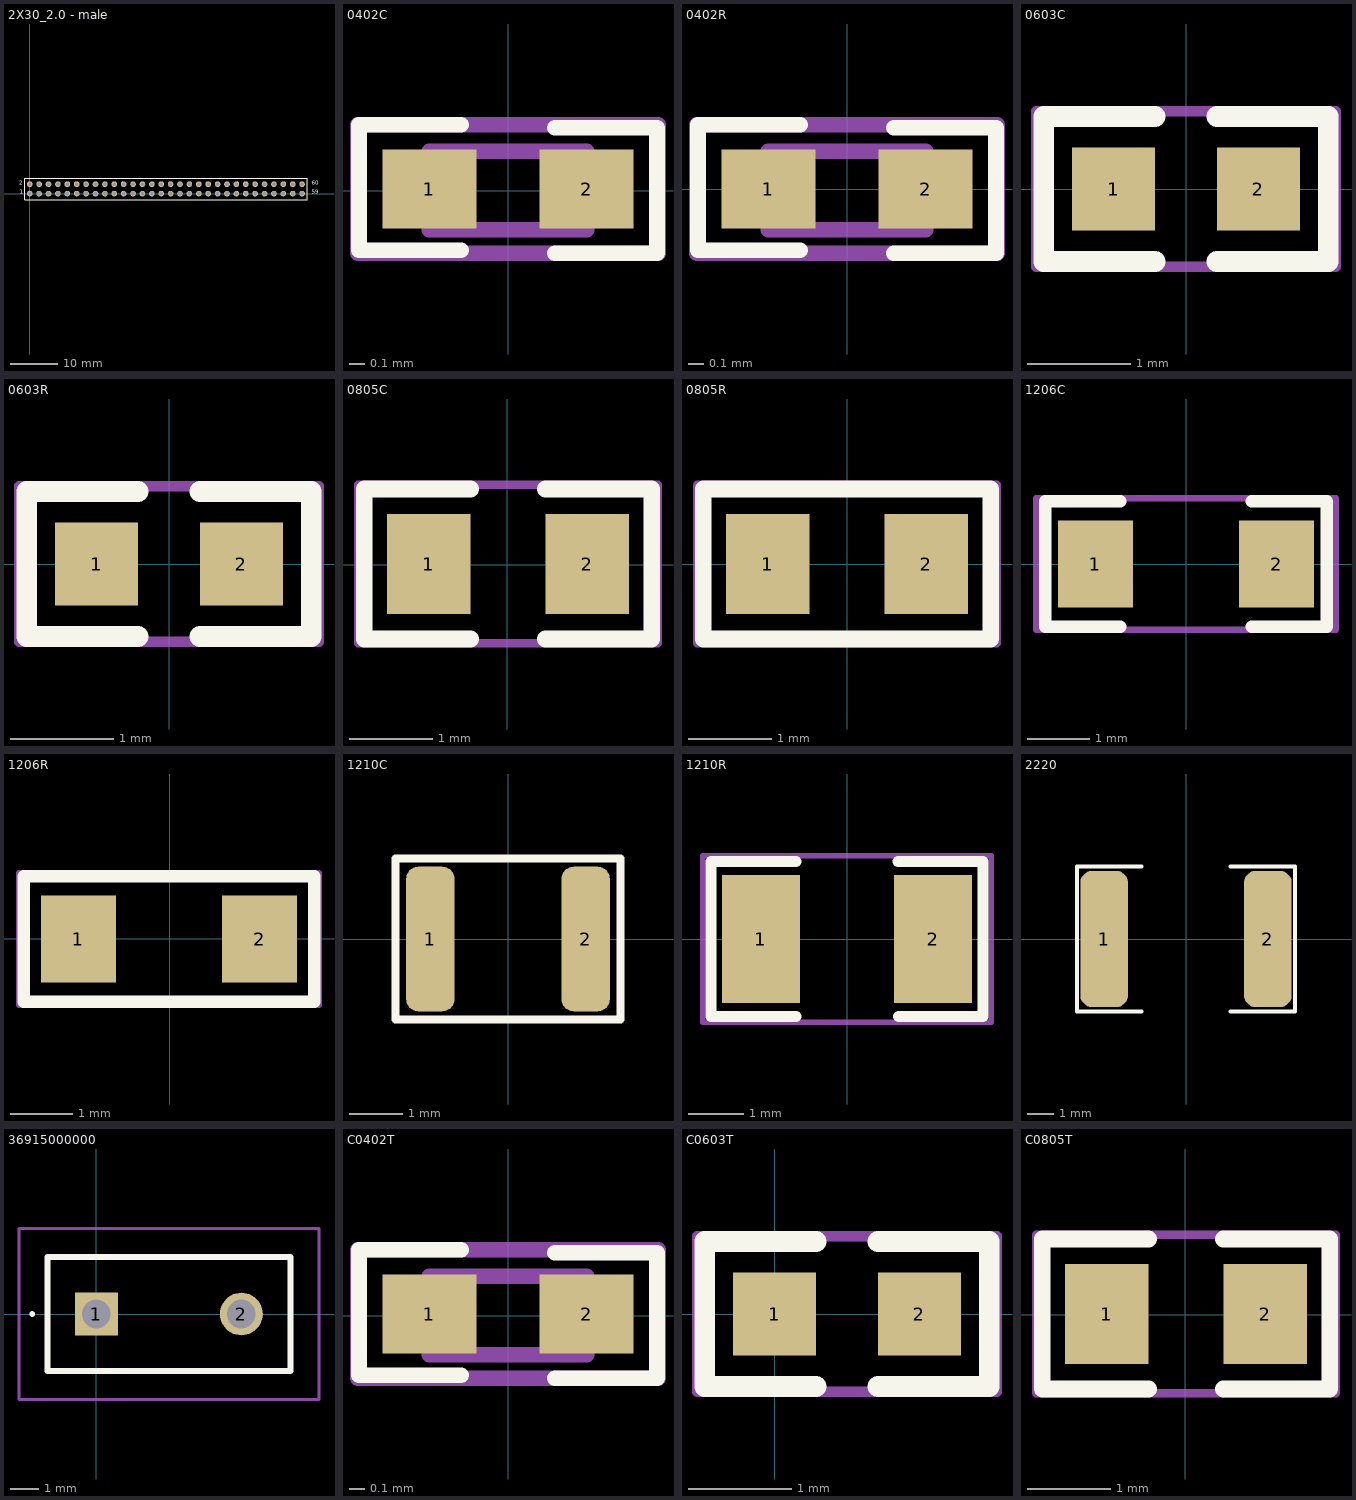
[diagram p0: the footprints below, top view; thin cyan lines are the x and y axes]
# Altium footprint library MISC82254-2.PcbLib: 93 footprints (part 1 of 6)
Each footprint in its own frame and in the unit in brackets; x right, y up, seen from the top. Pads: shape width x height; smd on the part's side, far side on the other; paste and mask are expansions set on the pad; w line width, h text height; cw(c..) or ccw(c..) is an arc to the next point about the centre after c.

## 2X30_2.0 - male [mm]
pads (60):
  round 1.2 hole 0.8: 1(0,0) 2(0,2) 3(2,0) 4(2,2) 5(4,0) 6(4,2) 7(6,0) 8(6,2) 9(8,0) 10(8,2) 11(10,0) 12(10,2) 13(12,0) 14(12,2) 15(14,0) 16(14,2) 17(16,0) 18(16,2) 19(18,0) 20(18,2) 21(20,0) 22(20,2) 23(22,0) 24(22,2) 25(24,0) 26(24,2) 27(26,0) 28(26,2) 29(28,0) 30(28,2) 31(30,0) 32(30,2) 33(32,0) 34(32,2) 35(34,0) 36(34,2) 37(36,0) 38(36,2) 39(38,0) 40(38,2) 41(40,0) 42(40,2) 43(42,0) 44(42,2) 45(44,0) 46(44,2) 47(46,0) 48(46,2) 49(48,0) 50(48,2) 51(50,0) 52(50,2) 53(52,0) 54(52,2) 55(54,0) 56(54,2) 57(56,0) 58(56,2) 59(58,0) 60(58,2)
Top Overlay:
  lines w0.254: -1.099,-1.308 -1.099,3.264 59.099,3.264 59.099,-1.308 -1.099,-1.308
  text "1" at -2.159,-0.381 h1.52
  text "2" at -2.286,1.524 h1.52
  text "60" at 60.071,1.524 h1.52
  text "59" at 60.071,-0.381 h1.52
3D body "HDR2.0-LI-2x15P.STEP": height 2.8, standoff -6.5, extent -1,-1 29,3
3D body "HDR2.0-LI-2x15P.STEP": height 2.8, standoff -6.5, extent 29,-1 59,3

## 0402C [mm]
pads (2):
  rect 0.6x0.5 smd mask+0.05: 1(-0.5,0.01) 2(0.5,0.01)
Top Overlay:
  lines w0.1: -0.298,-0.381 -0.949,-0.381 -0.949,0.419 -0.298,0.419 ; 0.298,-0.4 0.949,-0.4 0.949,0.4 0.298,0.4
Mechanical 13:
  lines w0.1: -0.5,-0.25 -0.5,0.25 0.5,0.25 0.5,-0.25 -0.5,-0.25
Mechanical 15:
  lines w0.1: -0.955,-0.4 0.955,-0.4 0.955,0.4 ; -0.955,-0.381 -0.955,0.419 0.955,0.419
3D body "GRM155R60G225ME15D.stp": height 0.55, standoff 0, extent -0.5,-0.25 0.5,0.25

## 0402R [mm]
pads (2):
  rect 0.6x0.5 smd mask+0.05: 1(-0.5,0) 2(0.5,0)
Top Overlay:
  lines w0.1: -0.298,-0.39 -0.949,-0.39 -0.949,0.41 -0.298,0.41 ; 0.298,-0.41 0.949,-0.41 0.949,0.39 0.298,0.39
Mechanical 13:
  lines w0.1: -0.5,-0.26 0.5,-0.26 0.5,0.24 -0.5,0.24 -0.5,-0.26
Mechanical 15:
  lines w0.1: -0.955,-0.41 0.955,-0.41 0.955,0.39 ; -0.955,-0.39 -0.955,0.41 0.955,0.41
3D body "CPF0402B100KE.stp": height 0.35, standoff 0, extent -0.5,-0.25 0.5,0.25

## 0603C [mm]
pads (2):
  rect 0.8x0.8 smd: 1(-0.7,0) 2(0.7,0)
Top Overlay:
  lines w0.2: -0.3,-0.7 -1.375,-0.7 -1.375,0.7 -0.3,0.7 ; 0.3,-0.7 1.375,-0.7 1.375,0.7 0.3,0.7
Mechanical 15:
  lines w0.1: -1.45,-0.75 1.45,-0.75 1.45,0.75 -1.45,0.75 -1.45,-0.75
3D body "C0603.step": height 0.8, standoff 0, extent -0.8,-0.4 0.8,0.4

## 0603R [mm]
pads (2):
  rect 0.8x0.8 smd: 1(-0.7,0) 2(0.7,0)
Top Overlay:
  lines w0.2: -0.3,-0.7 -1.375,-0.7 -1.375,0.7 -0.3,0.7 ; 0.3,-0.7 1.375,-0.7 1.375,0.7 0.3,0.7
Mechanical 15:
  lines w0.1: -1.45,-0.75 -1.45,0.75 1.45,0.75 1.45,-0.75 -1.45,-0.75
3D body "R0603.step": height 0.8, standoff 0, extent -0.8,-0.406 0.8,0.394

## 0805C [mm]
pads (2):
  rect 1x1.2 smd: 1(-0.94,0.007) 2(0.96,0.007)
Top Overlay:
  lines w0.2: -0.44,-0.893 -1.715,-0.893 -1.715,0.907 -0.44,0.907 ; 0.46,-0.893 1.735,-0.893 1.735,0.907 0.46,0.907
Mechanical 15:
  lines w0.1: -1.79,-0.943 1.81,-0.943 1.81,0.957 -1.79,0.957 -1.79,-0.943
3D body "GRM21B5C1H103JA01L.stp": height 1.45, standoff 0, extent -1,-0.625 1,0.625

## 0805R [mm]
pads (2):
  rect 1x1.2 smd: 1(-0.95,0) 2(0.95,0)
Top Overlay:
  lines w0.2: -1.725,-0.9 -1.725,0.9 1.725,0.9 1.725,-0.9 -1.725,-0.9
Mechanical 15:
  lines w0.1: -1.8,-0.95 -1.8,0.95 1.8,0.95 1.8,-0.95 -1.8,-0.95
3D body "CRGH0805F49K9.stp": height 0.65, standoff 0, extent -1,-0.637 1,0.637

## 1206C [mm]
pads (2):
  rect 1.2x1.4 smd: 1(-1.45,0) 2(1.45,0)
Top Overlay:
  lines w0.2: -1.051,-1 -2.25,-1 -2.25,1 -1.051,1 ; 1.051,-1 2.25,-1 2.25,1 1.051,1
Mechanical 15:
  lines w0.1: -2.4,-1.05 2.4,-1.05 2.4,1.05 -2.4,1.05 -2.4,-1.05
3D body "VJ1206A103JXATW1BC.stp": height 1.7, standoff 0, extent -1.6,-0.8 1.6,0.8

## 1206R [mm]
pads (2):
  rect 1.2x1.4 smd: 1(-1.459,-0.006) 2(1.441,-0.006)
Top Overlay:
  lines w0.2: -2.334,-1.006 2.316,-1.006 2.316,0.994 -2.334,0.994 -2.334,-1.006
Mechanical 15:
  lines w0.1: -2.409,-1.056 2.391,-1.056 2.391,1.044 -2.409,1.044 -2.409,-1.056
3D body "CRGH1206J2M0.stp": height 0.65, standoff 0, extent -1.55,-0.787 1.55,0.787

## 1210C [mm] "capacitor 1210 reflow soldering"
pads (2):
  rrect50% 0.9x2.7 smd: 1(-1.45,0) 2(1.45,0)
Top Overlay:
  lines w0.15: -2.1,-1.5 2.1,-1.5 2.1,1.5 -2.1,1.5 -2.1,-1.5
3D body "CAP1210.stp": height 0.92, standoff -0.02, extent -1.6,-1.25 1.6,1.25

## 1210R [mm]
pads (2):
  rect 1.4x2.3 smd: 1(-1.55,0) 2(1.55,0)
Top Overlay:
  lines w0.2: -0.915,-1.393 -2.45,-1.393 -2.45,1.393 -0.915,1.393 ; 0.915,1.393 2.45,1.393 2.45,-1.393 0.925,-1.393
Mechanical 15:
  lines w0.1: -2.6,-1.5 2.6,-1.5 2.6,1.5 -2.6,1.5 -2.6,-1.5
3D body "12105E103MAT2A.stp": height 0.94, standoff 0, extent -1.538,-1.263 1.662,1.237
3D body "CRCW12101R82FNEA.stp": height 0.6, standoff 0, extent -1.6,-1.25 1.6,1.25

## 2220 [mil]
height 110.24
pads (2):
  rrect50% 70x200 smd: 1(-120,0) 2(120,0)
Top Overlay:
  lines w5.91: -64.96,-106.3 -160,-106.3 -160,106.3 -64.96,106.3 ; 64.96,-106.3 160,-106.3 160,106.3 64.96,106.3
3D body: height 110.24, standoff 0, extent -120,-106.49 120,106.5

## 36915000000 [mm]
height 2.8
pads (2):
  rect 1.5x1.5 hole 1: 1(0,0)
  round 1.5 hole 1: 2(5.08,0)
Top Overlay:
  lines w0.1: -2.3,0 cw(c-2.25,0) -2.2,0 cw(c-2.25,0) -2.3,0
  lines w0.2: -1.71,-2 6.8,-2 6.8,2 -1.71,2 -1.71,-2
Mechanical 13:
  lines w0.1: -1.71,-2 6.79,-2 6.79,2 -1.71,2 -1.71,-2
Mechanical 15:
  lines w0.1: -2.71,-3 7.8,-3 7.8,3 -2.71,3 -2.71,-3
3D body "36915000000.stp": height 8.1, standoff -5, extent -1.71,-2 6.79,2

## C0402T [mm]
pads (2):
  rect 0.6x0.5 smd mask+0.05: 1(-0.5,0.01) 2(0.5,0.01)
Top Overlay:
  lines w0.1: -0.298,-0.381 -0.949,-0.381 -0.949,0.419 -0.298,0.419 ; 0.298,-0.4 0.949,-0.4 0.949,0.4 0.298,0.4
Mechanical 13:
  lines w0.1: -0.5,-0.25 0.5,-0.25 0.5,0.25 -0.5,0.25 -0.5,-0.25
Mechanical 15:
  lines w0.1: -0.955,-0.4 0.955,-0.4 0.955,0.4 ; -0.955,-0.381 -0.955,0.419 0.955,0.419
3D body "GRM155R60G225ME15D.stp": height 0.55, standoff 0, extent -0.5,-0.25 0.5,0.25

## C0603T [mm]
pads (2):
  rect 0.8x0.8 smd: 1(0,0) 2(1.4,0)
Top Overlay:
  lines w0.2: 0.4,-0.7 -0.675,-0.7 -0.675,0.7 0.4,0.7 ; 1,-0.7 2.075,-0.7 2.075,0.7 1,0.7
Mechanical 15:
  lines w0.1: -0.75,-0.75 -0.75,0.75 2.15,0.75 2.15,-0.75 -0.75,-0.75
3D body "C0603.step": height 0.8, standoff 0, extent -0.1,-0.4 1.5,0.4

## C0805T [mm]
pads (2):
  rect 1x1.2 smd: 1(-0.94,0.007) 2(0.96,0.007)
Top Overlay:
  lines w0.2: -0.44,-0.893 -1.715,-0.893 -1.715,0.907 -0.44,0.907 ; 0.46,-0.893 1.735,-0.893 1.735,0.907 0.46,0.907
Mechanical 15:
  lines w0.1: -1.79,-0.943 -1.79,0.957 1.81,0.957 1.81,-0.943 -1.79,-0.943
3D body "GRM21B5C1H103JA01L.stp": height 1.45, standoff 0, extent -1,-0.625 1,0.625